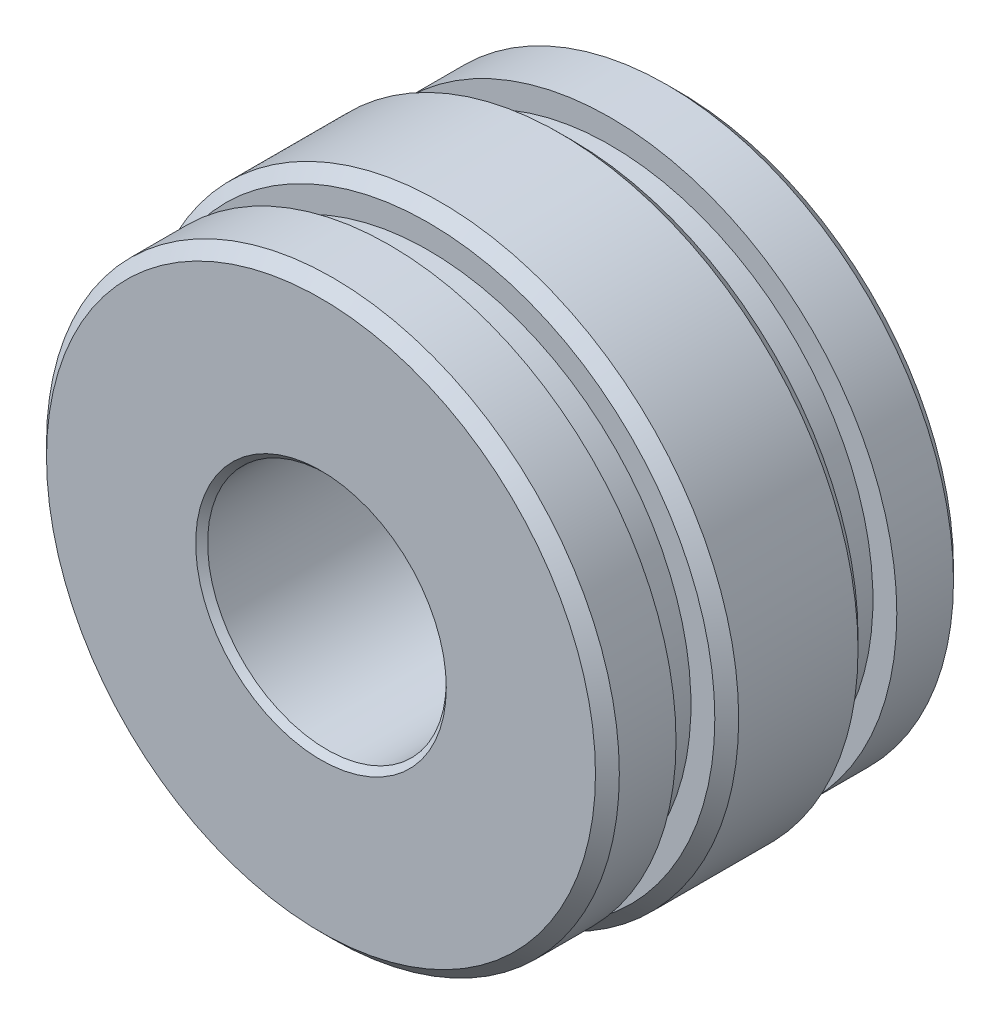
from build123d import *

# Parameters (mm, degrees)
SKETCH1_R           = 50
SKETCH1_R_2         = 20
BOSS_EXTRUDE1_DEPTH = 60
CUT_EXTRUDE1_START  = -42
SKETCH2_R           = 50
SKETCH2_R_2         = 44
CUT_EXTRUDE1_DEPTH  = 6.5
CUT_EXTRUDE2_START  = 11.5
SKETCH3_R           = 50
SKETCH3_R_2         = 44
CUT_EXTRUDE2_DEPTH  = 6.5
CUT_EXTRUDE3_START  = -12
SKETCH5_R           = 50
SKETCH5_R_2         = 48
CUT_EXTRUDE3_DEPTH  = 12
SKETCH6_R           = 50
SKETCH6_R_2         = 48
CUT_EXTRUDE4_DEPTH  = 12
CHAMFER1_SIZE       = 2
CHAMFER2_SIZE       = 1
CHAMFER3_SIZE       = 2


with BuildPart() as part:
    # Sketch1 → Boss-Extrude1 (new body)
    with BuildSketch(Plane.XY):
        Circle(SKETCH1_R)
        Circle(SKETCH1_R_2, mode=Mode.SUBTRACT)
    extrude(amount=BOSS_EXTRUDE1_DEPTH)

    # Sketch2 → Cut-Extrude1 (cut)
    with BuildSketch(Plane(origin=(0, 0, 0), x_dir=(-1, 0, 0), z_dir=(0, 0, -1)).offset(CUT_EXTRUDE1_START)):
        Circle(SKETCH2_R)
        Circle(SKETCH2_R_2, mode=Mode.SUBTRACT)
    extrude(amount=-CUT_EXTRUDE1_DEPTH, mode=Mode.SUBTRACT)

    # Sketch3 → Cut-Extrude2 (cut)
    with BuildSketch(Plane.XY.offset(CUT_EXTRUDE2_START)):
        Circle(SKETCH3_R)
        with Locations(Location((0, 0, 0), (0, 0, 180))):
            Circle(SKETCH3_R_2, mode=Mode.SUBTRACT)
    extrude(amount=CUT_EXTRUDE2_DEPTH, mode=Mode.SUBTRACT)

    # Sketch5 → Cut-Extrude3 (cut)
    with BuildSketch(Plane.XY.offset(60).offset(CUT_EXTRUDE3_START)):
        Circle(SKETCH5_R)
        Circle(SKETCH5_R_2, mode=Mode.SUBTRACT)
    extrude(amount=CUT_EXTRUDE3_DEPTH, mode=Mode.SUBTRACT)

    # Sketch6 → Cut-Extrude4 (cut)
    with BuildSketch(Plane(origin=(0, 0, 0), x_dir=(-1, 0, 0), z_dir=(0, 0, -1))):
        Circle(SKETCH6_R)
        with Locations(Location((0, 0, 0), (0, 0, 180))):
            Circle(SKETCH6_R_2, mode=Mode.SUBTRACT)
    extrude(amount=-CUT_EXTRUDE4_DEPTH, mode=Mode.SUBTRACT)

    # Chamfer1
    chamfer1_edges = [part.edges().sort_by_distance(p)[0] for p in [
        (-48, 0, 60),
        (-48, 0, 0),
    ]]
    chamfer(chamfer1_edges, length=CHAMFER1_SIZE)

    # Chamfer2
    chamfer2_edges = [part.edges().sort_by_distance(p)[0] for p in [
        (-20, 0, 0),
        (-20, 0, 60),
    ]]
    chamfer(chamfer2_edges, length=CHAMFER2_SIZE)

    # Chamfer3
    chamfer3_edges = [part.edges().sort_by_distance(p)[0] for p in [
        (-50, 0, 42),
        (-50, 0, 18),
    ]]
    chamfer(chamfer3_edges, length=CHAMFER3_SIZE)


solid = part.part
